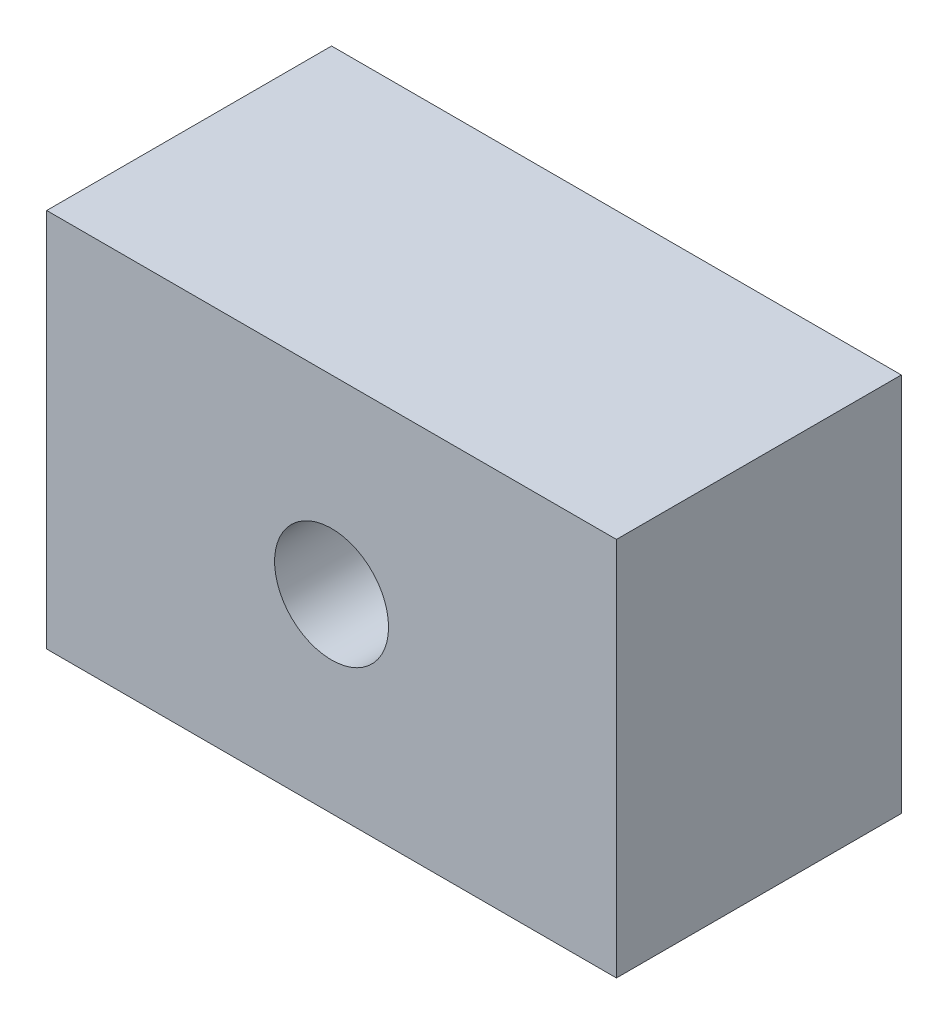
SolidWorks part; units mm, degrees
ref_plane "Front Plane" through (0, 0, 0) normal (0, 0, 1) x (1, 0, 0)
ref_plane "Top Plane" through (0, 0, 0) normal (0, 1, 0) x (1, 0, 0)
ref_plane "Right Plane" through (0, 0, 0) normal (1, 0, 0) x (0, 0, -1)
sketch "Sketch1" plane through (0, 0, 0) normal (0, 0, 1) x (1, 0, 0)
  line L1 (-15, 10) -> (15, 10)
  line L2 (-15, 10) -> (-15, -10)
  line L3 (-15, -10) -> (15, -10)
  line L4 (15, 10) -> (15, -10)
  line L5 (-15, 10) -> (15, -10) construction
  line L6 (-15, -10) -> (15, 10) construction
  point P0 (0, 0)
  dimension "D1" = 20
  dimension "D2" = 30
extrude "Boss-Extrude1" add sketch "Sketch1" along normal blind 15
sketch "Sketch2" plane through (0, 0, 15) normal (0, 0, 1) x (1, 0, 0)
  circle A0 centre (0, 0) radius 3
  dimension "D1" = 6
extrude "Cut-Extrude1" cut sketch "Sketch2" against normal through all both and the other way through all
